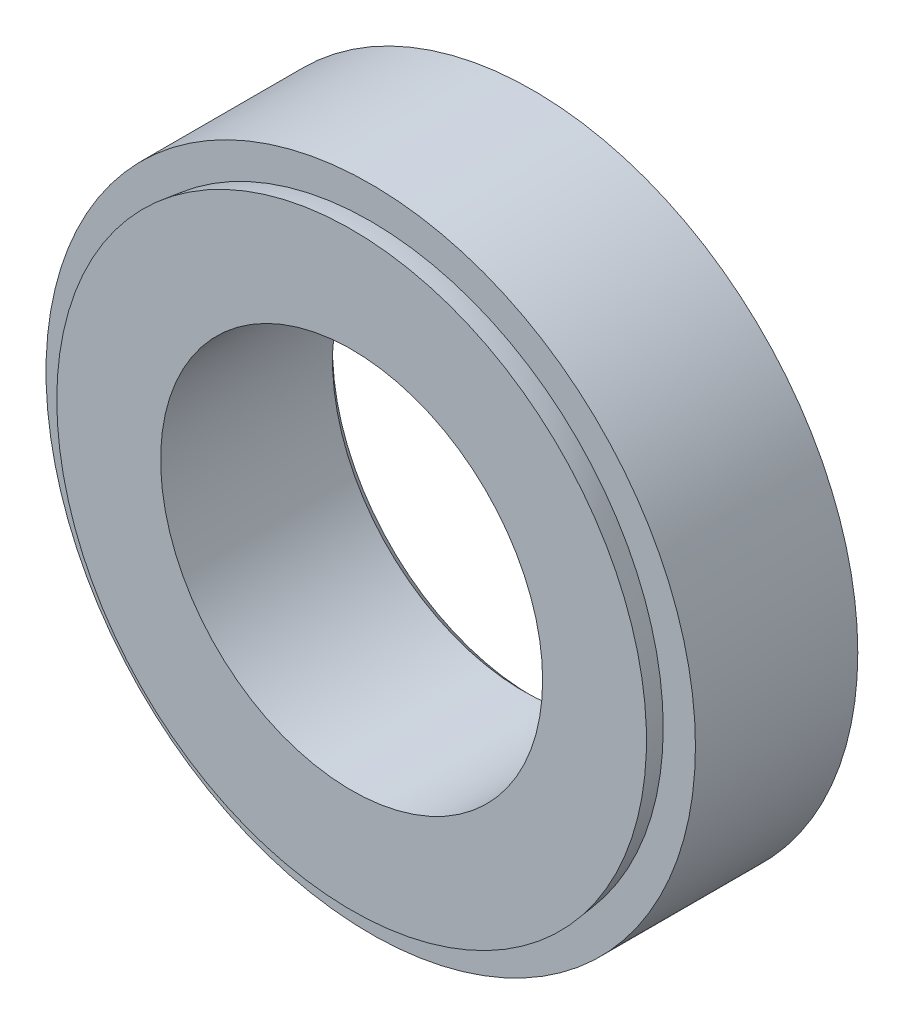
from build123d import *

# Parameters (mm, degrees)
SKETCH_1_R          = 34
EXTRUDE_1_DEPTH     = 19
SKETCH_3_R          = 20
CUT_EXTRUDE_1_DEPTH = 52.701063819
CHAMFER_1_SIZE      = 1


with BuildPart() as part:
    # 草图1 → 凸台-拉伸1 (new body)
    with BuildSketch(Plane.XY):
        Circle(SKETCH_1_R)
    extrude(amount=EXTRUDE_1_DEPTH)

    # 草图2 → 切除-旋转1 (revolve, cut)
    with BuildSketch(Plane(origin=(0, 0, 0), x_dir=(1, 0, 0), z_dir=(0, 1, 0)), mode=Mode.PRIVATE) as cut_revolve_1_sk:
        with BuildLine():
            Line((-34, -17), (-30.626132632, -17))
            ThreePointArc((-30.626132632, -17), (-30.765967048, -17.997991107), (-30.873289426, -19))
            Line((-30.873289426, -19), (-34, -19))
            Line((-34, -19), (-34, -17))
        make_face()
    revolve(cut_revolve_1_sk.sketch.rotate(Axis((0, 0, 19), (0, 0, -1)), 180), axis=Axis((0, 0, 19), (0, 0, -1)), mode=Mode.SUBTRACT)

    # 草图3 → 切除-拉伸1 (cut, through all)
    with BuildSketch(Plane.XY.offset(19)):
        Circle(SKETCH_3_R)
    extrude(amount=-CUT_EXTRUDE_1_DEPTH, mode=Mode.SUBTRACT)

    # 倒角1
    chamfer_1_edges = [part.edges().sort_by_distance(p)[0] for p in [
        (-20, 0, 0),
    ]]
    chamfer(chamfer_1_edges, length=CHAMFER_1_SIZE)


solid = part.part
